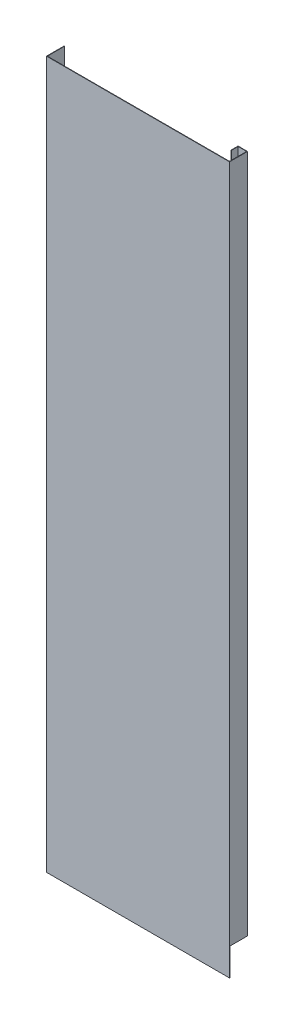
SolidWorks part; units mm, degrees
ref_plane "Front Plane" through (0, 0, 0) normal (0, 0, 1) x (1, 0, 0)
ref_plane "Top Plane" through (0, 0, 0) normal (0, 1, 0) x (1, 0, 0)
ref_plane "Right Plane" through (0, 0, 0) normal (1, 0, 0) x (0, 0, -1)
sketch "Sketch3" plane through (0, 0, 0) normal (0, 1, 0) x (1, 0, 0)
  line L0 (0, 40) -> (0, 0)
  line L1 (0, 0) -> (425, 0)
  line L2 (425, 0) -> (425, 40)
  line L3 (425, 40) -> (405, 40)
  line L4 (405, 40) -> (405, 25)
  dimension "D1" = 40
  dimension "D2" = 425
  dimension "D3" = 40
  dimension "D4" = 20
  dimension "D5" = 15
extrude "Extrude-Thin1" add sketch "Sketch3" along normal blind 1649 thin
sketch "Sketch5" plane through (0, 0, -41) normal (0, 0, -1) x (-1, 0, 0)
  line L0 (-404, 1649) -> (-404, 0) construction
  line L1 (-426, 0) -> (-404, 0)
  line L2 (-426, 0) -> (-426, 64)
  line L3 (-426, 64) -> (-404, 64)
  line L4 (-404, 0) -> (-404, 64)
  dimension "D1" = 64
extrude "Cut-Extrude2" cut sketch "Sketch5" against normal up to surface (41 mm away) up to face at (212.5, 824.5, 0)
